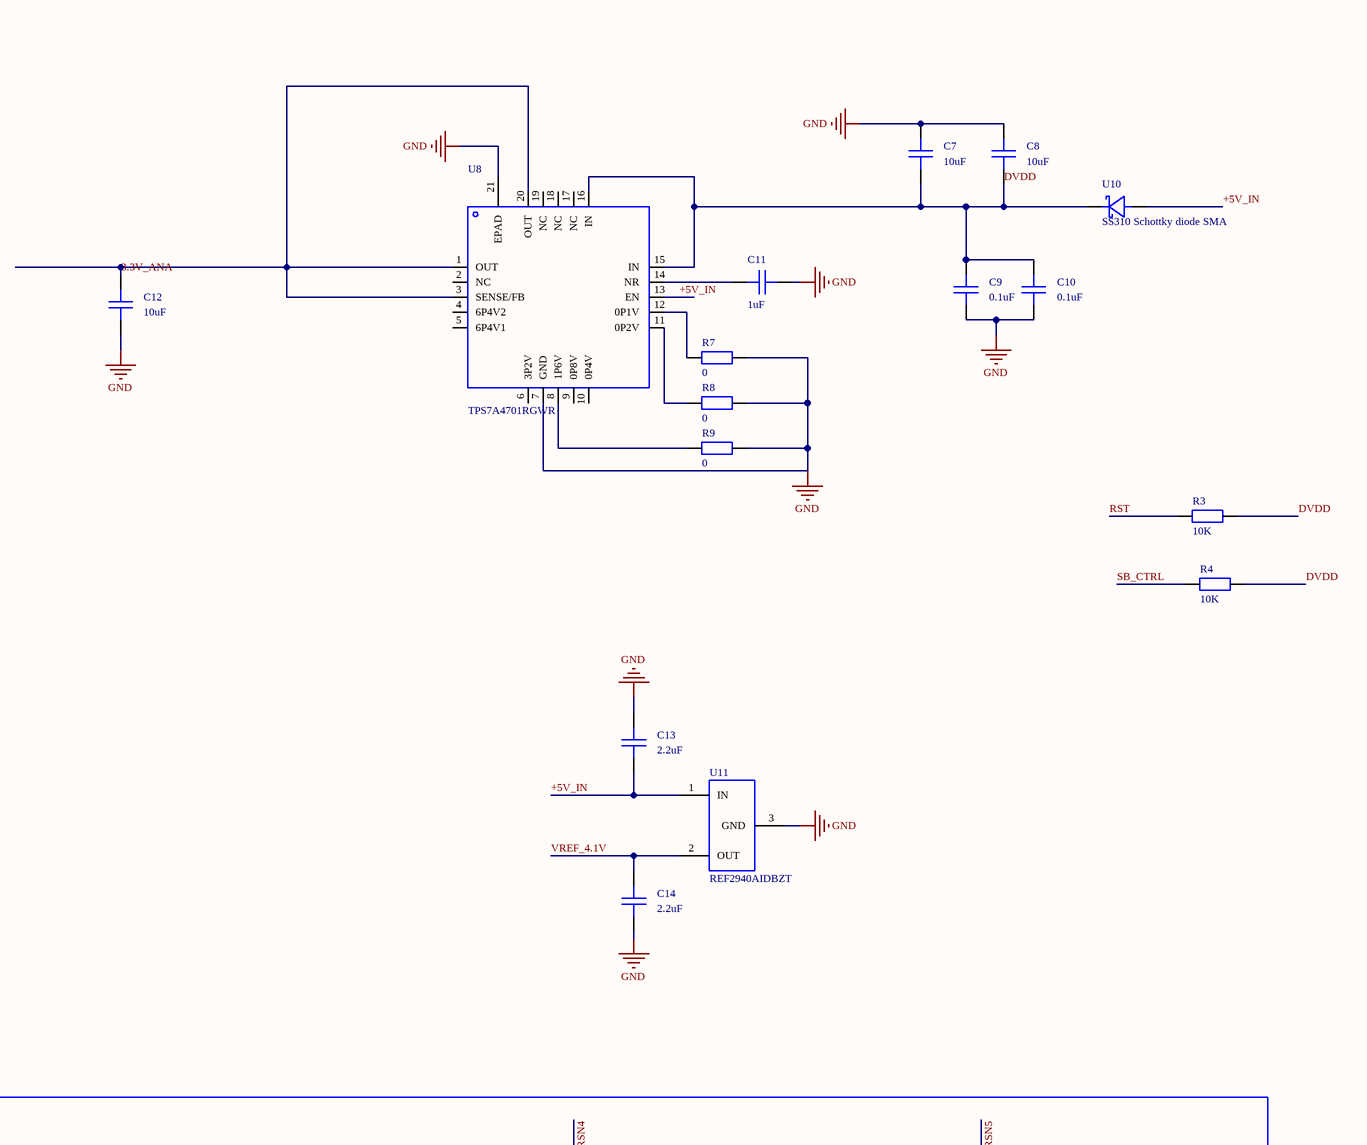
[diagram p0: MISC49910-3.schdoc, top left]
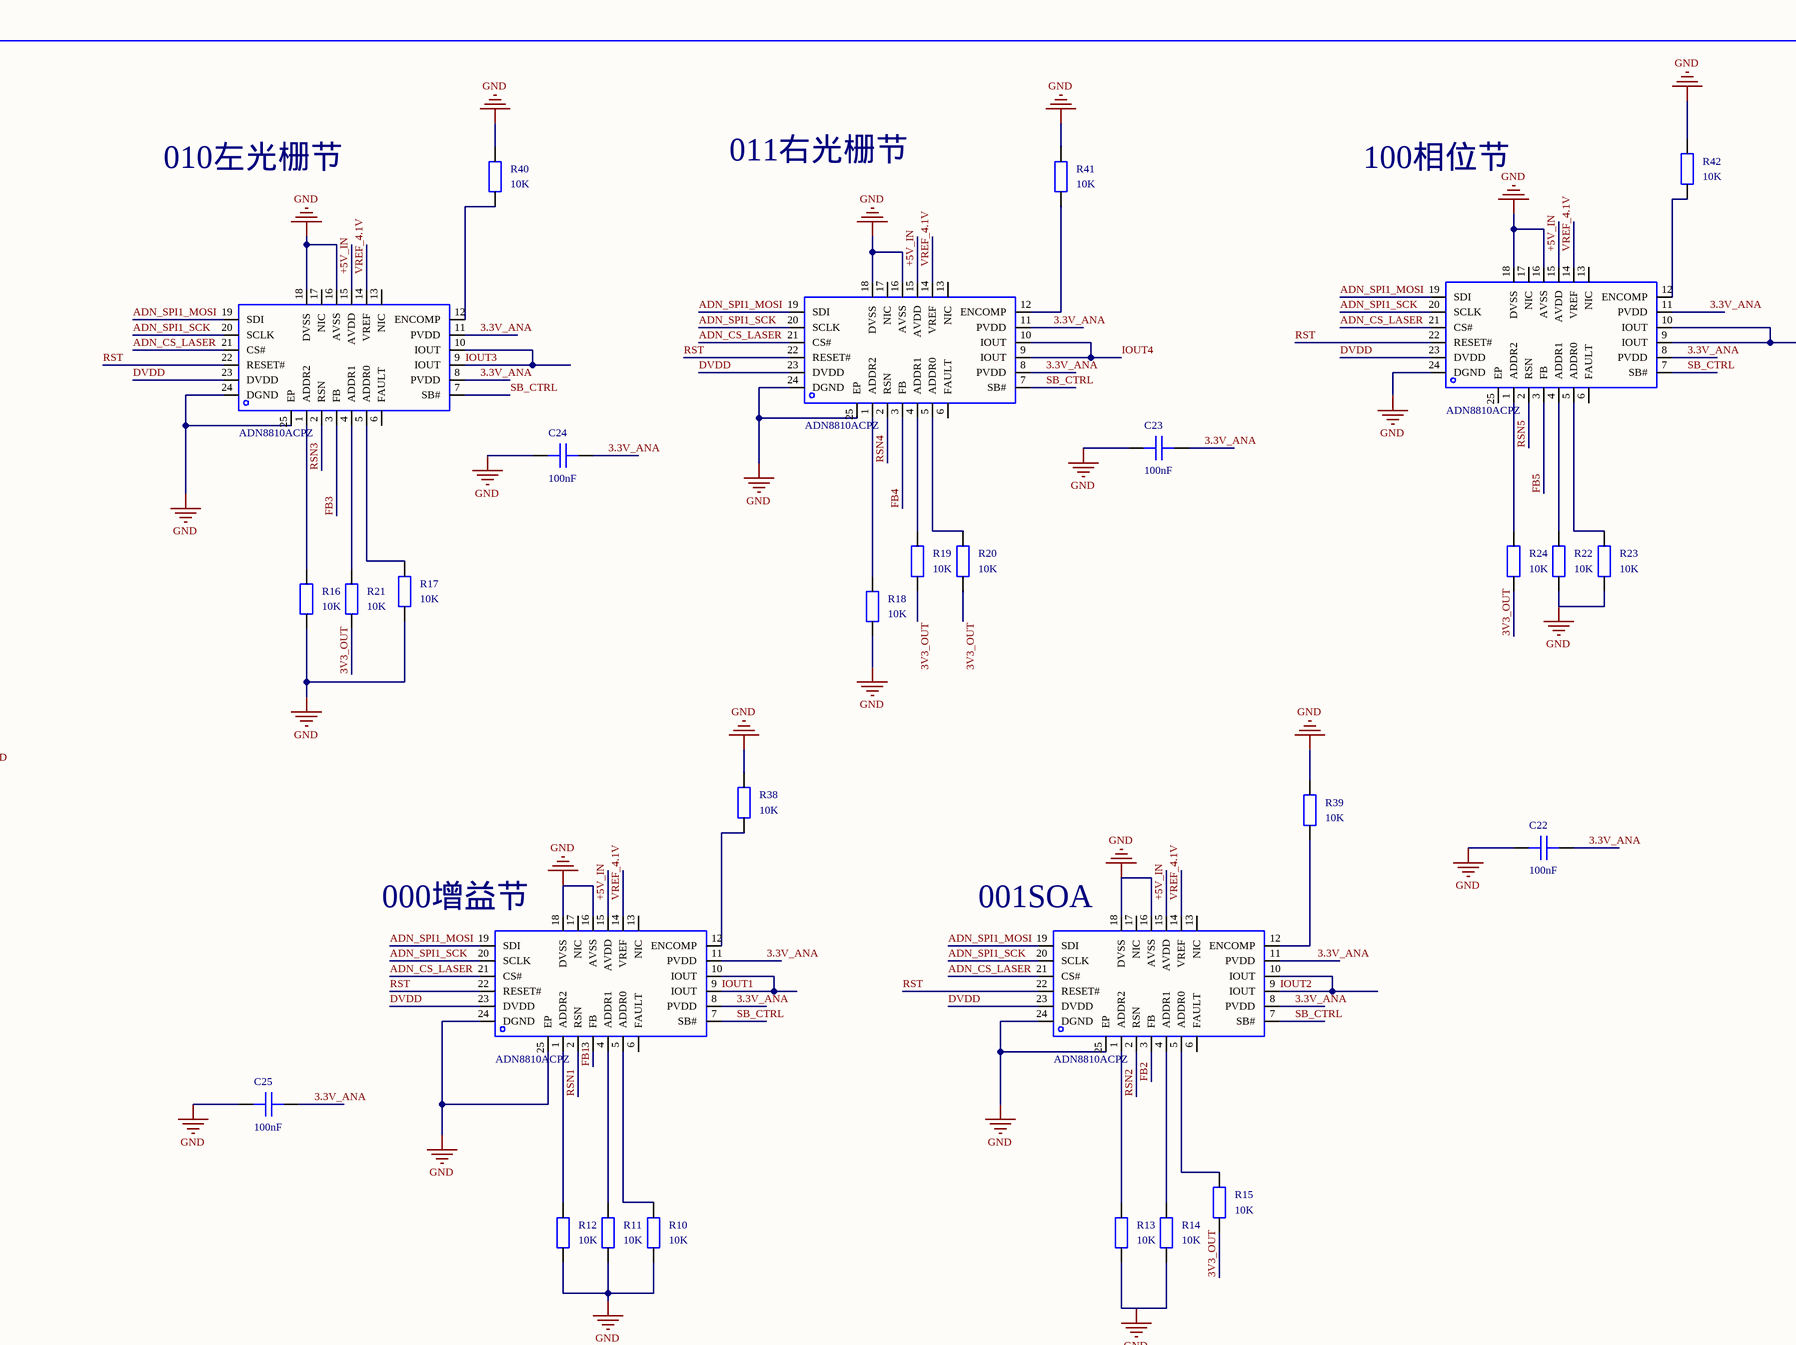
[diagram p1: MISC49910-3.schdoc, top middle]
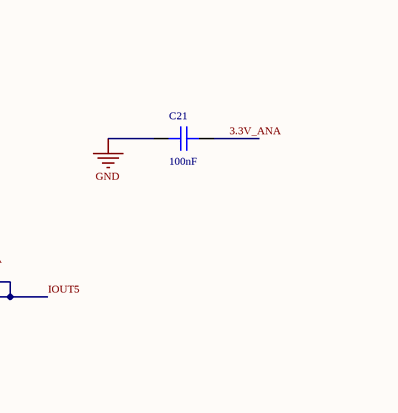
[diagram p2: MISC49910-3.schdoc, top right]
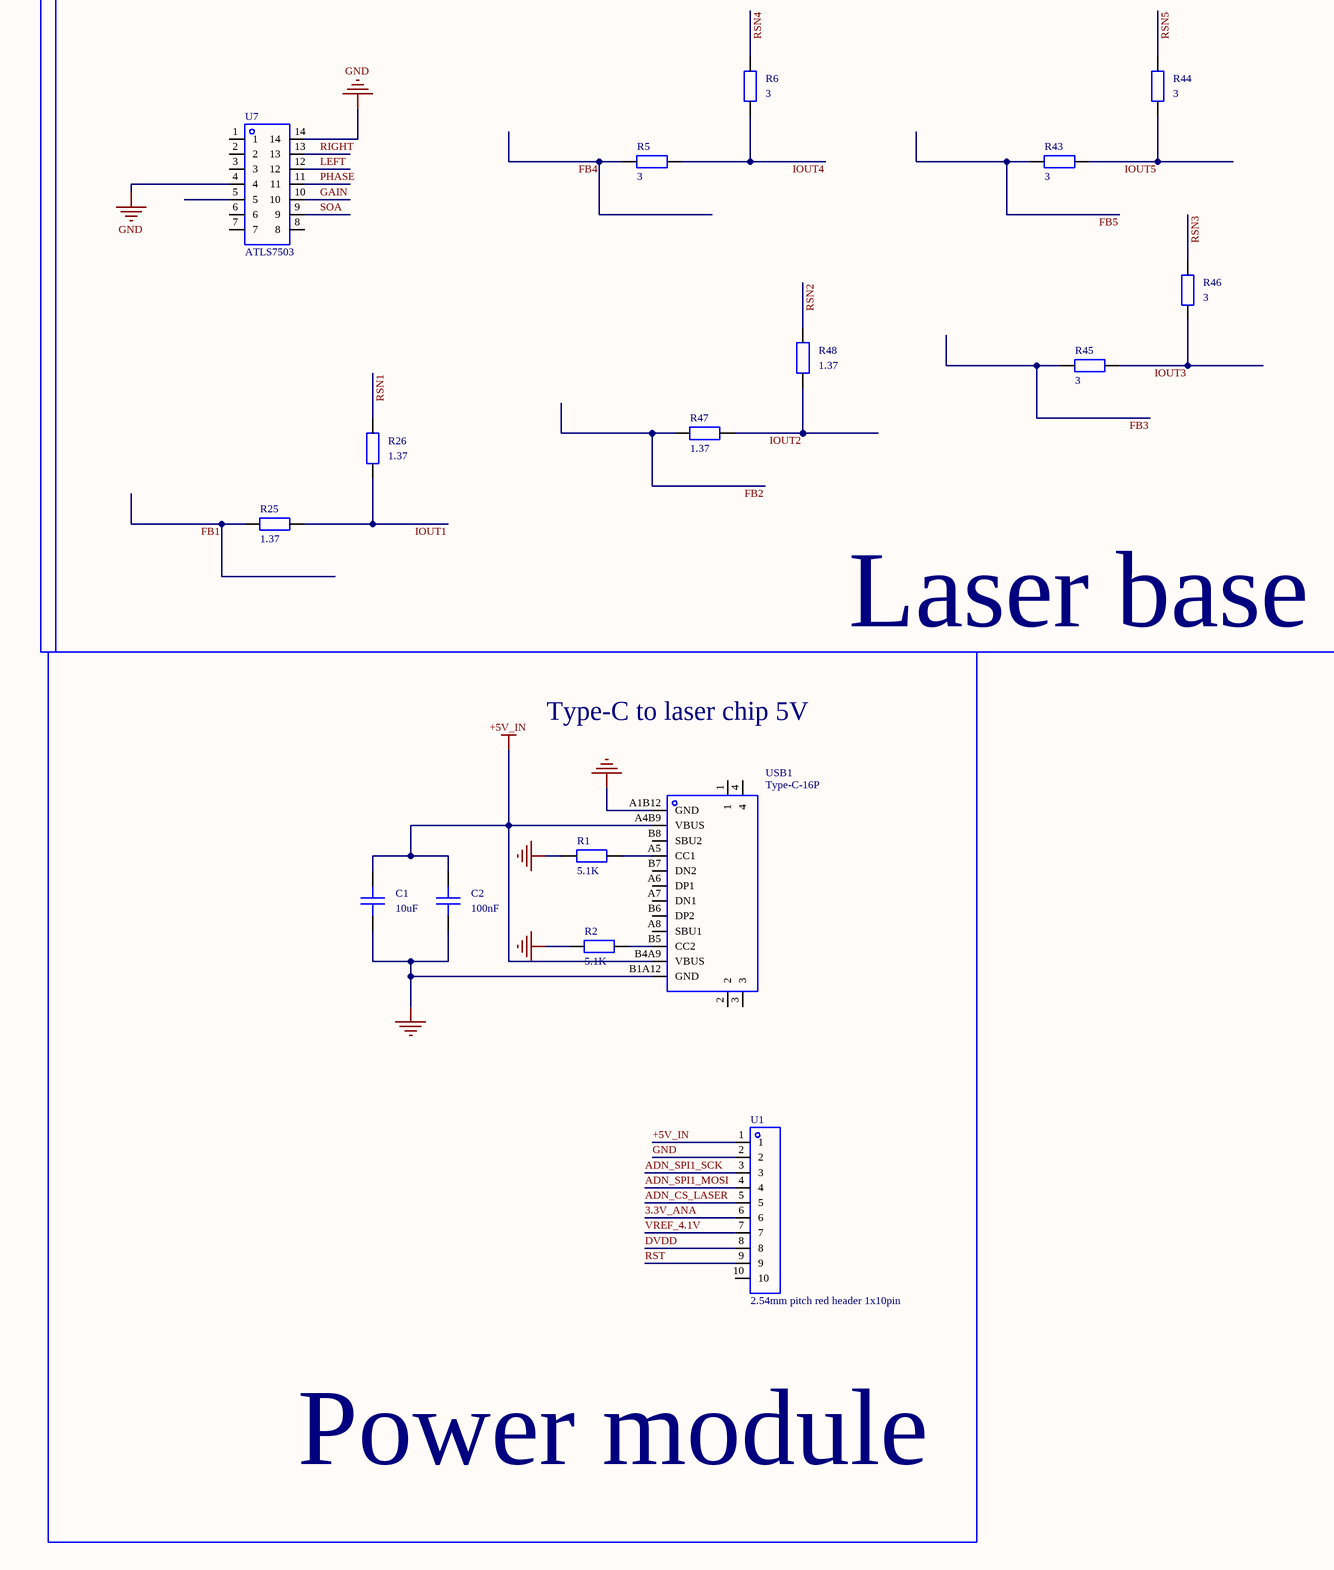
[diagram p3: MISC49910-3.schdoc, centre left]
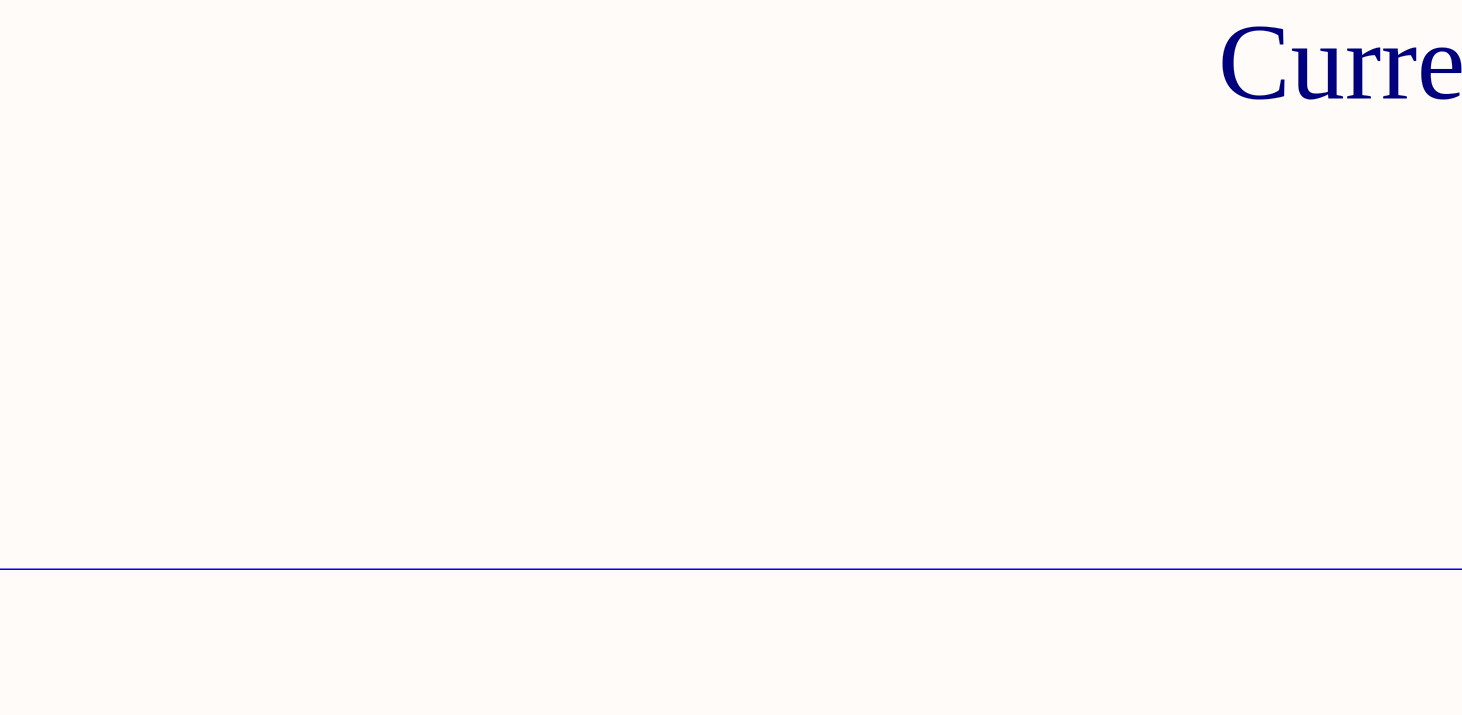
[diagram p4: MISC49910-3.schdoc, centre middle]
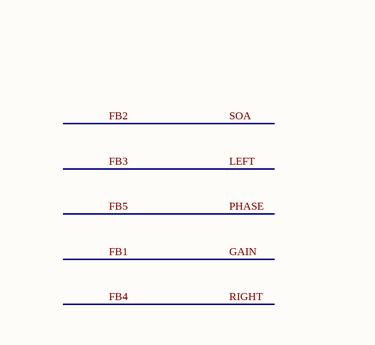
[diagram p5: MISC49910-3.schdoc, bottom right]
# Altium project MISC49910.PrjPcb
1 sheet, 63 parts. Net scope: global (net labels, ports and power ports of the same name join across sheets).
Board file: MISC49910.pcbdoc

## Sheet MISC49910-3.schdoc
size 635 x 635 mm; @Board Name: MISC49910; @Create Time: 17:30:08; @Page Count: 1; @Page No: 1; @Schematic Name: MISC49910; @Update Time: 17:30:08; Size: A4; Version: V1.0; @Project Name: MISC49910; @Update Date: 2026-04-20; @Create Date: 2026-04-20

### Parts
000增益节  ADN8810ACPZ  [LFCSP-24_L4.0-W4.0-P0.50-BL-EP2.3]
001SOA  ADN8810ACPZ  [LFCSP-24_L4.0-W4.0-P0.50-BL-EP2.3]
010左光栅节  ADN8810ACPZ  [LFCSP-24_L4.0-W4.0-P0.50-BL-EP2.3]
011右光栅节  ADN8810ACPZ  [LFCSP-24_L4.0-W4.0-P0.50-BL-EP2.3]
100相位节  ADN8810ACPZ  [LFCSP-24_L4.0-W4.0-P0.50-BL-EP2.3]
C1  10uF  [C0402]
C2  100nF  [C0402]
C7  10uF  [C0603]
C8  10uF  [C0603]
C9  0.1uF  [C0603]
C10  0.1uF  [C0603]
C11  1uF  [C0603]
C12  10uF  [C0603]
C13  2.2uF  [C0603]
C14  2.2uF  [C0603]
C21  100nF  [C0603]
C22  100nF  [C0603]
C23  100nF  [C0603]
C24  100nF  [C0603]
C25  100nF  [C0603]
R1  5.1K  [R0603]
R2  5.1K  [R0603]
R3  10K  [R0603]
R4  10K  [R0603]
R5  3  [R0603]
R6  3  [R0603]
R7  0  [R0603]
R8  0  [R0603]
R9  0  [R0603]
R10  10K  [R0603]
R11  10K  [R0603]
R12  10K  [R0603]
R13  10K  [R0603]
R14  10K  [R0603]
R15  10K  [R0603]
R16  10K  [R0603]
R17  10K  [R0603]
R18  10K  [R0603]
R19  10K  [R0603]
R20  10K  [R0603]
R21  10K  [R0603]
R22  10K  [R0603]
R23  10K  [R0603]
R24  10K  [R0603]
R25  1.37  [R0603]
R26  1.37  [R0603]
R38  10K  [R0603]
R39  10K  [R0603]
R40  10K  [R0603]
R41  10K  [R0603]
R42  10K  [R0603]
R43  3  [R0603]
R44  3  [R0603]
R45  3  [R0603]
R46  3  [R0603]
R47  1.37  [R0603]
R48  1.37  [R0603]
U1  2.54mm pitch red header 1x10pin  [HDR-TH_10P-P2.54-V-F-2]
U7  ATLS7503  [HDR-SMD_14P-P1.27-V-F-R2-C7-LS4.8]
U8  TPS7A4701RGWR  [VQFN-20_L5.0-W5.0-P0.65-TL-EP]
U10  SS310 Schottky diode SMA  [SMA_L4.3-W2.6-LS5.1-R-RD]
U11  REF2940AIDBZT  [SOT-23-3_L2.9-W1.3-P1.90-LS2.4-BR]
USB1  Type-C-16P  [USB-C-SMD_GT-USB-7010E]

### Blocks framed on the sheet
Current source module: 000增益节 001SOA 010左光栅节 011右光栅节 100相位节 C7-C14 C21-C25 R3 R4 R7-R24 R38-R42 U8 U10 U11
Laser base: R5 R6 R25 R26 R43-R48 U7

### Nets
+5V_IN: 000增益节.15(AVDD) 001SOA.15(AVDD) 010左光栅节.15(AVDD) 011右光栅节.15(AVDD) 100相位节.15(AVDD) C1.2 C2.2 C13.1 U1.1 U8.13(EN) U10.1(A) U11.1(IN) USB1.A4B9(VBUS) USB1.B4A9(VBUS)
GND: 000增益节.16(AVSS) 000增益节.18(DVSS) 000增益节.24(DGND) 000增益节.25(EP) 001SOA.16(AVSS) 001SOA.18(DVSS) 001SOA.24(DGND) 001SOA.25(EP) 010左光栅节.16(AVSS) 010左光栅节.18(DVSS) 010左光栅节.24(DGND) 010左光栅节.25(EP) 011右光栅节.16(AVSS) 011右光栅节.18(DVSS) 011右光栅节.24(DGND) 011右光栅节.25(EP) 100相位节.16(AVSS) 100相位节.18(DVSS) 100相位节.24(DGND) C1.1 C2.1 C7.2 C8.2 C9.1 C10.1 C11.1 C12.1 C13.2 C14.1 C21.2 C22.2 C23.2 C24.2 C25.2 R1.1 R2.1 R7.2 R8.2 R9.2 R10.1 R11.1 R12.1 R13.1 R14.1 R16.1 R17.1 R18.1 R22.1 R23.1 R38.2 R39.2 R40.2 R41.2 R42.2 U1.2 U7.4 U7.14 U8.7(GND) U8.21(EPAD) U11.3(GND) USB1.A1B12(GND) USB1.B1A12(GND)
3.3V_ANA: 000增益节.8(PVDD) 000增益节.11(PVDD) 001SOA.8(PVDD) 001SOA.11(PVDD) 010左光栅节.8(PVDD) 010左光栅节.11(PVDD) 011右光栅节.8(PVDD) 011右光栅节.11(PVDD) 100相位节.8(PVDD) 100相位节.11(PVDD) C12.2 C21.1 C22.1 C23.1 C24.1 C25.1 U1.6 U8.1(OUT) U8.3(SENSE/FB) U8.20(OUT)
3V3_OUT: R15.1 R19.1 R20.1 R21.1 R24.1
ADN_CS_LASER: 000增益节.21(CS#) 001SOA.21(CS#) 010左光栅节.21(CS#) 011右光栅节.21(CS#) 100相位节.21(CS#) U1.5
ADN_SPI1_MOSI: 000增益节.19(SDI) 001SOA.19(SDI) 010左光栅节.19(SDI) 011右光栅节.19(SDI) 100相位节.19(SDI) U1.4
ADN_SPI1_SCK: 000增益节.20(SCLK) 001SOA.20(SCLK) 010左光栅节.20(SCLK) 011右光栅节.20(SCLK) 100相位节.20(SCLK) U1.3
DVDD: 000增益节.23(DVDD) 001SOA.23(DVDD) 010左光栅节.23(DVDD) 011右光栅节.23(DVDD) 100相位节.23(DVDD) C7.1 C8.1 C9.2 C10.2 R3.2 R4.2 U1.8 U8.15(IN) U8.16(IN) U10.2(K)
FB1: 000增益节.3(FB) R25.2 U7.10  [also labelled GAIN]
FB2: 001SOA.3(FB) R47.2 U7.9  [also labelled SOA]
FB3: 010左光栅节.3(FB) R45.2 U7.12  [also labelled LEFT]
FB4: 011右光栅节.3(FB) R5.2 U7.13  [also labelled RIGHT]
FB5: 100相位节.3(FB) R43.2 U7.11  [also labelled PHASE]
IOUT1: 000增益节.9(IOUT) 000增益节.10(IOUT) R25.1 R26.2
IOUT2: 001SOA.9(IOUT) 001SOA.10(IOUT) R47.1 R48.2
IOUT3: 010左光栅节.9(IOUT) 010左光栅节.10(IOUT) R45.1 R46.2
IOUT4: 011右光栅节.9(IOUT) 011右光栅节.10(IOUT) R5.1 R6.2
IOUT5: 100相位节.9(IOUT) 100相位节.10(IOUT) R43.1 R44.2
RSN1: 000增益节.2(RSN) R26.1
RSN2: 001SOA.2(RSN) R48.1
RSN3: 010左光栅节.2(RSN) R46.1
RSN4: 011右光栅节.2(RSN) R6.1
RSN5: 100相位节.2(RSN) R44.1
RST: 000增益节.22(RESET#) 001SOA.22(RESET#) 010左光栅节.22(RESET#) 011右光栅节.22(RESET#) 100相位节.22(RESET#) R3.1 U1.9
SB_CTRL: 000增益节.7(SB#) 001SOA.7(SB#) 010左光栅节.7(SB#) 011右光栅节.7(SB#) 100相位节.7(SB#) R4.1
VREF_4.1V: 000增益节.14(VREF) 001SOA.14(VREF) 010左光栅节.14(VREF) 011右光栅节.14(VREF) 100相位节.14(VREF) C14.2 U1.7 U11.2(OUT)
Net000增益节_1: 000增益节.1(ADDR2) R12.2
Net000增益节_4: 000增益节.4(ADDR1) R11.2
Net000增益节_5: 000增益节.5(ADDR0) R10.2
Net000增益节_12: 000增益节.12(ENCOMP) R38.1
Net001SOA_1: 001SOA.1(ADDR2) R13.2
Net001SOA_4: 001SOA.4(ADDR1) R14.2
Net001SOA_5: 001SOA.5(ADDR0) R15.2
Net001SOA_12: 001SOA.12(ENCOMP) R39.1
Net010左光栅节_1: 010左光栅节.1(ADDR2) R16.2
Net010左光栅节_4: 010左光栅节.4(ADDR1) R21.2
Net010左光栅节_5: 010左光栅节.5(ADDR0) R17.2
Net010左光栅节_12: 010左光栅节.12(ENCOMP) R40.1
Net011右光栅节_1: 011右光栅节.1(ADDR2) R18.2
Net011右光栅节_4: 011右光栅节.4(ADDR1) R19.2
Net011右光栅节_5: 011右光栅节.5(ADDR0) R20.2
Net011右光栅节_12: 011右光栅节.12(ENCOMP) R41.1
Net100相位节_1: 100相位节.1(ADDR2) R24.2
Net100相位节_4: 100相位节.4(ADDR1) R22.2
Net100相位节_5: 100相位节.5(ADDR0) R23.2
Net100相位节_12: 100相位节.12(ENCOMP) R42.1
NetC11_2: C11.2 U8.14(NR)
NetR1_2: R1.2 USB1.A5(CC1)
NetR2_2: R2.2 USB1.B5(CC2)
NetR7_1: R7.1 U8.12(0P1V)
NetR8_1: R8.1 U8.11(0P2V)
NetR9_1: R9.1 U8.8(1P6V)

Not connected (* = marked no-connect by the designer): 000增益节 6(FAULT) 13(NIC) 17(NIC); 001SOA 6(FAULT) 13(NIC) 17(NIC); 010左光栅节 6(FAULT) 13(NIC) 17(NIC); 011右光栅节 6(FAULT) 13(NIC) 17(NIC); 100相位节 6(FAULT) 13(NIC) 17(NIC) 25(EP); U1 10; U7 1 2 3 5 6 7 8; U8 2(NC) 4(6P4V2) 5(6P4V1) 6(3P2V) 9(0P8V) 10(0P4V) 17(NC) 18(NC) 19(NC); USB1 1 2 3 4 A6(DP1) A7(DN1) A8(SBU1) B6(DP2) B7(DN2) B8(SBU2)

### Notes on the sheet
- Type-C to laser chip 5V
- Power module
- 2025-12-16
- Schematic
- Board
- Sheet
- P1
- Drawn
- Reviewed
- Revision
- Size
- A4
- page 1 Total 1

### Library data of the parts
000增益节 = ADN8810ACPZ: Output current: 300mA;; Manufacturer: ADI(亚德诺); AddInBom: yes; ModelId: fa197dd414874ad2bc21045e91d88c960819f05c4eef4c71ace90d822a990e87; ModelName: LFCSP-24_L4.0-W4.0-H0.8-P0.50; ModelTransform: 157.48,157.48,0,90,0,0,0,0,0; Device: ADN8810ACPZ; Symbol: ADN8810ACPZ; FootprintName: LFCSP-24_L4.0-W4.0-P0.50-BL-EP2.3; LCSC Part Name: 12位高输出电流源; SupplierPart: C579232; ManufacturerPart: ADN8810ACPZ; Supplier Footprint: LFCSP-24(4x4); JLCPCB Part Class: Extended Part; Datasheet: example.com/datasheet/ADN8810ACPZ/607009.html; Supplier: LCSC; ConvertToPcb: yes; Type: Current source; Output Current: 300mA; Operating Temperature: -40℃~+85℃
001SOA 010左光栅节 011右光栅节 100相位节 = ADN8810ACPZ: Output current: 300mA;; Manufacturer: ADI(亚德诺); 3D Model: fa197dd414874ad2bc21045e91d88c960819f05c4eef4c71ace90d822a990e87; 3D Model Transform: 157.48,157.48,0,90,0,0,0,0,0; AddInBom: yes; ModelName: LFCSP-24_L4.0-W4.0-H0.8-P0.50; Device: ADN8810ACPZ; Symbol: ADN8810ACPZ; LCSC Part Name: 12位高输出电流源; Supplier Part: C579232; Manufacturer Part: ADN8810ACPZ; Supplier Footprint: LFCSP-24(4x4); JLCPCB Part Class: Extended Part; Datasheet: example.com/datasheet/ADN8810ACPZ/607009.html; Supplier: LCSC; Type: Current source; Output Current: 300mA; Operating Temperature: -40℃~+85℃; FootprintName: LFCSP-24_L4.0-W4.0-P0.50-BL-EP2.3; ConvertToPcb: yes
C1 C2 = AC0402KRX7R7BB103: Capacitance: 10nF; accuracy: ±10%; rated voltage: 16V; temperature coefficient: X7R;; Manufacturer: YAGEO(国巨); AddInBom: yes; ModelId: 36a51122f27c49738f86b3bfa98863e00819f05c4eef4c71ace90d822a990e87; ModelName: C0402_L1.0-W0.5-H0.5; ModelTransform: 39.37,19.685,0,0,0,0,0,0,0; Device: AC0402KRX7R7BB103; Symbol: AC0402KRX7R7BB103; FootprintName: C0402; LCSC Part Name: 10nF ±10% 16V; ManufacturerPart: AC0402KRX7R7BB103; Supplier Footprint: 0402; JLCPCB Part Class: Extended Part; Datasheet: example.com/datasheet/AC0402KRX7R7BB103/773628.html; Supplier: LCSC; ConvertToPcb: yes; Tolerance: ±10%; Voltage Rating: 16V; Temperature Coefficient: X7R
  C1: Value: 10uF
  C2: Value: 100nF
C7-C10 = CAP_0603: Symbol: Capacitance; ConvertToPcb: yes; ModelId: 13237225da8613e4; ModelName: C0603_L1.6-W0.8-H0.8; ModelTransform: 0,0,0,0,0,0,0,0,0; Device: CAP_0603; FootprintName: C0603; AddInBom: yes; Supplier Footprint: 0603
  C7 C8: Value: 10uF
  C9 C10: Value: 0.1uF
C11-C14 C21-C25 = CAP_0603: Symbol: Capacitance; 3D Model: ac125912035d415993ca9572d50418b10819f05c4eef4c71ace90d822a990e87; 3D Model Transform: 62.992,31.496,0,0,0,0,0,0,0; ConvertToPcb: yes; ModelName: C0603_L1.6-W0.8-H0.8; Device: CAP_0603; Supplier Footprint: 0603; FootprintName: C0603; AddInBom: yes
  C11: Value: 1uF
  C12: Value: 10uF
  C13 C14: Value: 2.2uF
  C21-C25: Value: 100nF
R1 R2 = Res_0603: Symbol: Resistor; ConvertToPcb: yes; ModelId: 03cd5122016561a3; ModelTransform: 0,0,0,0,0,0,0,0,0; Device: Res_0603; Value: 5.1K; FootprintName: R0603; AddInBom: yes; Supplier Footprint: 0603; ModelName: R0603
R3 R4 = Res_0603: Symbol: Resistor; ConvertToPcb: yes; ModelId: fc143cca1e79419f9cd78b61e9279f080819f05c4eef4c71ace90d822a990e87; ModelTransform: 31.8897,63.7794,0,90,0,0,0,0,0; Device: Res_0603; FootprintName: R0603; AddInBom: yes; Supplier Footprint: 0603; Value: 10K; ModelName: R0603
R5-R26 R38-R48 = Res_0603: Symbol: Resistor; 3D Model: fc143cca1e79419f9cd78b61e9279f080819f05c4eef4c71ace90d822a990e87; 3D Model Transform: 31.8897,63.7794,0,90,0,0,0,0,0; ConvertToPcb: yes; Device: Res_0603; Supplier Footprint: 0603; FootprintName: R0603; AddInBom: yes; ModelName: R0603
  R5 R6 R43-R46: Value: 3
  R7-R9: Value: 0
  R10-R24 R38-R42: Value: 10K
  R25 R26 R47 R48: Value: 1.37
U1 = 间距2.54mm红色排母座1x10pin: AddInBom: yes; ModelId: 08a5ee31ec6747838a696d2ac093ffa40819f05c4eef4c71ace90d822a990e87; ModelName: HDR-TH_10P-P2.54-F-LI-1X10P; ModelTransform: 1009.87987,100,0,0,0,0,0,0,-125.984; Device: 2.54mm pitch red header 1x10pin; Symbol: 2.54MM pitch red header 1X10PIN; FootprintName: HDR-TH_10P-P2.54-V-F-2; LCSC Part Name: 间距2.54mm红色排母座1x10pin; SupplierPart: C9900015504; ManufacturerPart: 间距2.54mm红色排母座1x10pin; Supplier Footprint: 间距2.54MM单排母座红色(1*10P）; JLCPCB Part Class: Extended Part; Supplier: LCSC; ConvertToPcb: yes
U7 = HEADER7X2B: AddInBom: yes; ModelId: 15ced11fe4204b93ba29cc074fdc91ed0819f05c4eef4c71ace90d822a990e87; ModelName: HDR-SMD_14P-P1.27-F-LS-2X7P; ModelTransform: 365.747,188.976,0,0,0,0,0,0,0; Device: HEADER7X2B; Symbol: HEADER7X2B; Manufacturer Part: ATLS7503; FootprintName: HDR-SMD_14P-P1.27-V-F-R2-C7-LS4.8; LCSC Part Name: HEADER7X2B; SupplierPart: C9900007473; Supplier Footprint: HEADER7X2B; JLCPCB Part Class: Extended Part; Supplier: LCSC; ConvertToPcb: yes
U8 = TPS7A4701RGWR: Output type: adjustable; working voltage: 35V; output voltage: 1.4V~34V; output current: 1A; power supply rejection ratio (PSRR): 78dB@(1kHz); output polarity: positive;; Manufacturer: TI(德州仪器); AddInBom: yes; Voltage Dropout: 307mV@(1A); Noise: 4uVrms; Number of Outputs: 1; ModelId: eab1241f334749fa99541b9dbcc896380819f05c4eef4c71ace90d822a990e87; ModelName: VQFN-20_L5.0-W5.0-H1.0-P0.65; ModelTransform: 197.6374,197.6374,0,0,0,0,-0.006,0.006,0; Device: TPS7A4701RGWR; Symbol: TPS7A4701RGWR; FootprintName: VQFN-20_L5.0-W5.0-P0.65-TL-EP; LCSC Part Name: 具有使能功能的 1A、36V、低噪声、高 PSRR、低压降稳压器; SupplierPart: C90084; ManufacturerPart: TPS7A4701RGWR; Supplier Footprint: VQFN-20-EP(5x5); JLCPCB Part Class: Extended Part; Supplier: LCSC; ConvertToPcb: yes; Output Type: Adjustable; Voltage - Supply: 35V; Output Voltage: 1.4V~34V; Output Current: 1A; Power Supply Rejection Ratio (PSRR): 78dB@(1kHz); standby current: -; Features: Overcurrent protection; Operating Temperature: -40℃~+125℃@(Tj); Output Configuration: Positive
U10 = SS310肖特基二极管SMA: AddInBom: yes; ModelId: a03465a937202642; ModelTransform: 0,0,0,0,0,0,0,0,0; Device: SS310 Schottky diode SMA; Symbol: SS310 Schottky diode SMA; FootprintName: SMA_L4.3-W2.6-LS5.1-R-RD; LCSC Part Name: SS310肖特基二极管SMA; SupplierPart: C9900014981; ManufacturerPart: SS310肖特基二极管SMA; Supplier Footprint: SS310SMA110V; JLCPCB Part Class: Extended Part; Supplier: LCSC; ConvertToPcb: yes; ModelName: SMA_L4.3-W2.6-LS5.1-R-RD
U11 = REF2940AIDBZT: Output type: fixed; input voltage: 4.146V~5.5V; output voltage: 4.096V; output current: 25mA; accuracy: ±2%;; Manufacturer: TI(德州仪器); AddInBom: yes; Temperature Coefficient: 100ppm/℃; Reference Type: Series; Supply Current: 59uA; Noise - 1/10Hz to 10Hz: 45uVp-p; Noise - 10Hz to 10kHz: 128uVrms; ModelId: c62791f0466c4ae2a892c056b845b0ca0819f05c4eef4c71ace90d822a990e87; ModelName: SOT-23-3P_L2.9-W1.3-H1.0-LS2.4-P0.95; ModelTransform: 98.425,114.173,0,180,0,0,0.0005,-0.0005,0; Device: REF2940AIDBZT; Symbol: REF2940AIDBZT; FootprintName: SOT-23-3_L2.9-W1.3-P1.90-LS2.4-BR; LCSC Part Name: REF2940AIDBZT; SupplierPart: C111864; ManufacturerPart: REF2940AIDBZT; Supplier Footprint: SOT-23; JLCPCB Part Class: Extended Part; Supplier: LCSC; ConvertToPcb: yes; Output Type: Fixed; Input Voltage: 4.146V~5.5V; Output Voltage: 4.096V; Output Current: 25mA; Tolerance: ±2%; Operating Temperature: -40℃~+125℃@(Ta)
USB1 = Type-C-16P: AddInBom: yes; ModelId: 5afd3849e9c642128e878b8e27a760ba0819f05c4eef4c71ace90d822a990e87; ModelTransform: 351.9678,304.33,0,0,0,0,0,-43.307,-35.433; Device: Type-C-16P; Symbol: TYPE-C-16P; FootprintName: USB-C-SMD_GT-USB-7010E; LCSC Part Name: Type-C-16P; SupplierPart: C9900216560; ManufacturerPart: Type-C-16P; Supplier Footprint: SMD; JLCPCB Part Class: Extended Part; Supplier: LCSC; ConvertToPcb: yes; ModelName: USB-C-SMD_GT-USB-7010E